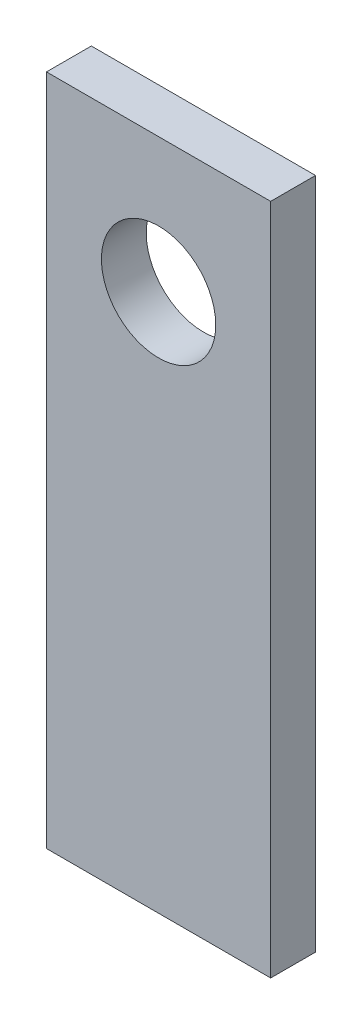
from build123d import *

# Parameters (mm, degrees)
SKETCH_1_W          = 50
SKETCH_1_H          = 150
EXTRUDE_1_DEPTH     = 5
CUT_EXTRUDE_1_REACH = 81.687
SKETCH_2_R          = 12.75


with BuildPart() as part:
    # 草图1 → 凸台-拉伸1 (new, symmetric)
    with BuildSketch(Plane.XY):
        Rectangle(SKETCH_1_W, SKETCH_1_H)
    extrude(amount=EXTRUDE_1_DEPTH, both=True)

    # 草图2 → 切除-拉伸1 (cut, up to next)
    with BuildSketch(Plane.XY.offset(5), mode=Mode.PRIVATE) as cut_extrude_1_sk1:
        with Locations((0, 45)):
            Circle(SKETCH_2_R)
    cut_extrude_1_tool1 = extrude(cut_extrude_1_sk1.sketch, amount=-CUT_EXTRUDE_1_REACH, mode=Mode.PRIVATE) & part.part
    add(cut_extrude_1_tool1.solids().sort_by_distance((0, 45, 5))[0], mode=Mode.SUBTRACT)


solid = part.part
